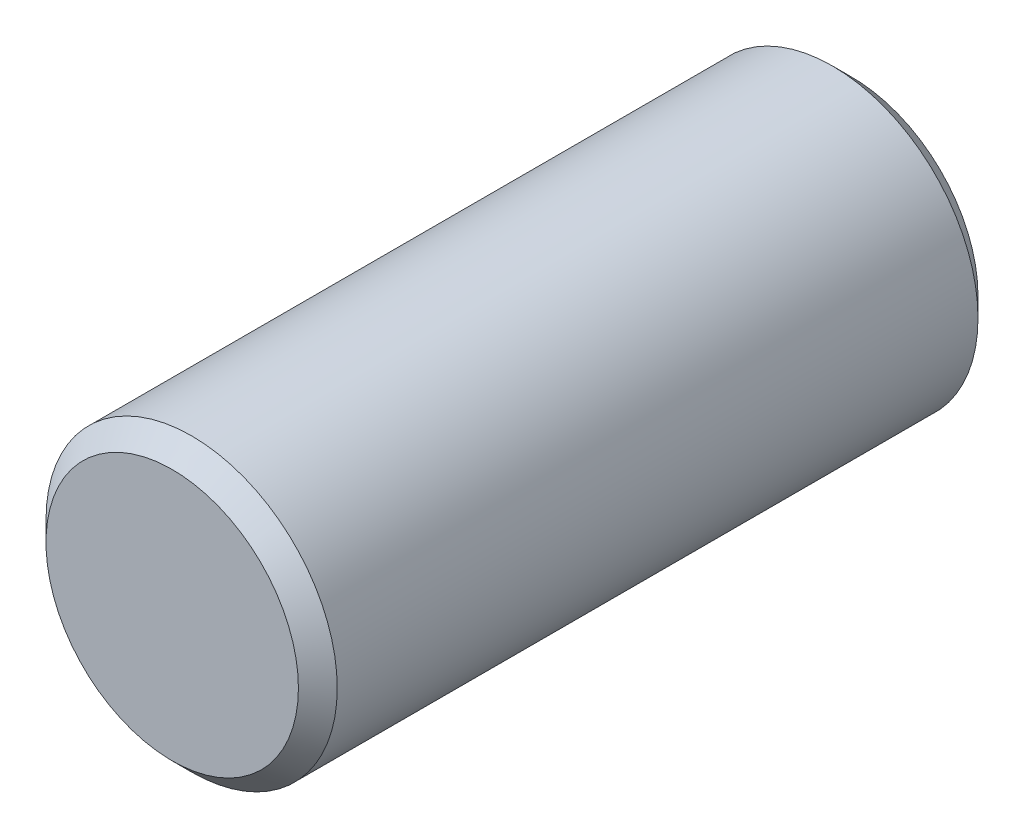
SolidWorks part; units mm, degrees
ref_plane "Front Plane" through (0, 0, 0) normal (0, 0, 1) x (1, 0, 0)
ref_plane "Top Plane" through (0, 0, 0) normal (0, 1, 0) x (1, 0, 0)
ref_plane "Right Plane" through (0, 0, 0) normal (1, 0, 0) x (0, 0, -1)
sketch "Sketch2" plane through (0, 0, 0) normal (0, 0, 1) x (1, 0, 0)
  circle A0 centre (-3.0591, 37.272) radius 1.5 construction
  circle A1 centre (-3.0591, 37.272) radius 1.5
extrude "Boss-Extrude2" add sketch "Sketch2" along normal blind 7
chamfer "Chamfer1" distance 0.2 angle 45 2 edges at (-1.5591, 37.272, 0) (-1.5591, 37.272, 7)
